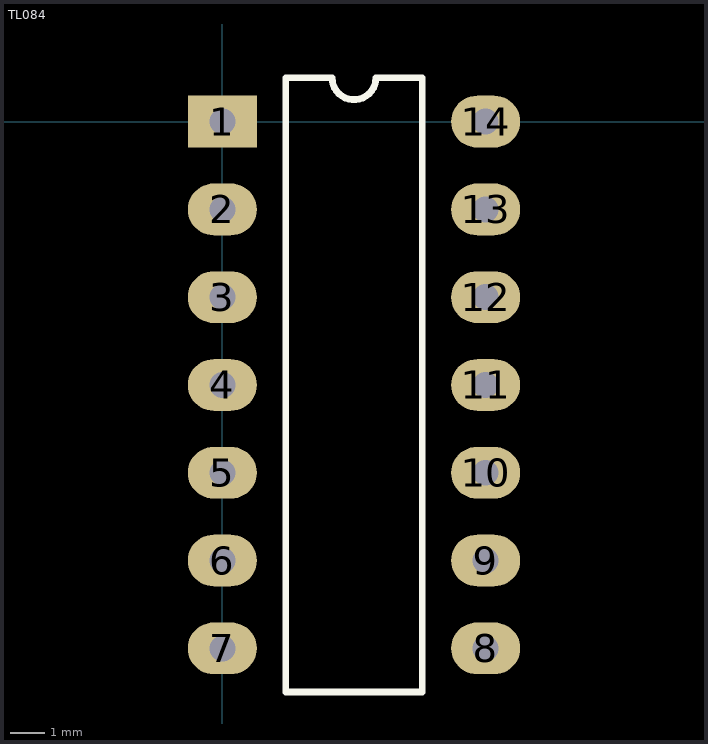
[diagram p0: the footprints below, top view; thin cyan lines are the x and y axes]
# Altium footprint library MISC89340-16.PcbLib: 2 footprints
Each footprint in its own frame and in the unit in brackets; x right, y up, seen from the top. Pads: shape width x height; smd on the part's side, far side on the other; paste and mask are expansions set on the pad; w line width, h text height; cw(c..) or ccw(c..) is an arc to the next point about the centre after c.

## PCBComponent_1 [mm]

## TL084 [mm]
pads (14):
  rect 2x1.5 hole 0.75: 1(0,0)
  oval 2x1.5 hole 0.75: 2(0,-2.54) 3(0,-5.08) 4(0,-7.62) 5(0,-10.16) 6(0,-12.7) 7(0,-15.24) 8(7.62,-15.24) 9(7.62,-12.7) 10(7.62,-10.16) 11(7.62,-7.62) 12(7.62,-5.08) 13(7.62,-2.54) 14(7.62,0)
Top Overlay:
  lines w0.2: 1.835,-16.51 1.835,1.27 3.175,1.27 ccw(c3.81,1.27) 4.445,1.27 5.785,1.27 5.785,-16.51 1.835,-16.51